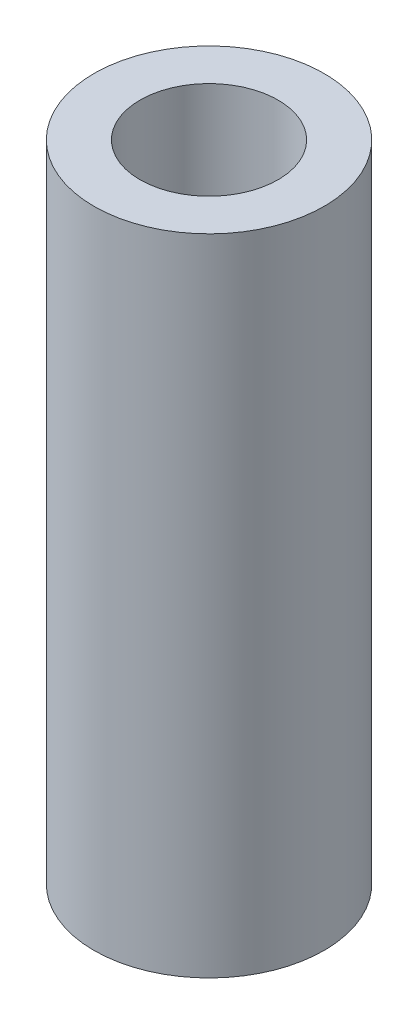
SolidWorks part; units mm, degrees
material "6061 合金"
ref_plane "前视基准面" through (0, 0, 0) normal (0, 0, 1) x (1, 0, 0)
ref_plane "上视基准面" through (0, 0, 0) normal (0, 1, 0) x (1, 0, 0)
ref_plane "右视基准面" through (0, 0, 0) normal (1, 0, 0) x (0, 0, -1)
other "Configuration Table"
sketch "草图1" plane through (0, 0, 0) normal (0, 1, 0) x (1, 0, 0)
  circle A0 centre (0, 0) radius 1.5
  circle A1 centre (0, 0) radius 2.5
  dimension "D1" = 3
  dimension "D2" = 5
extrude "凸台-拉伸1" add sketch "草图1" along normal blind 14
